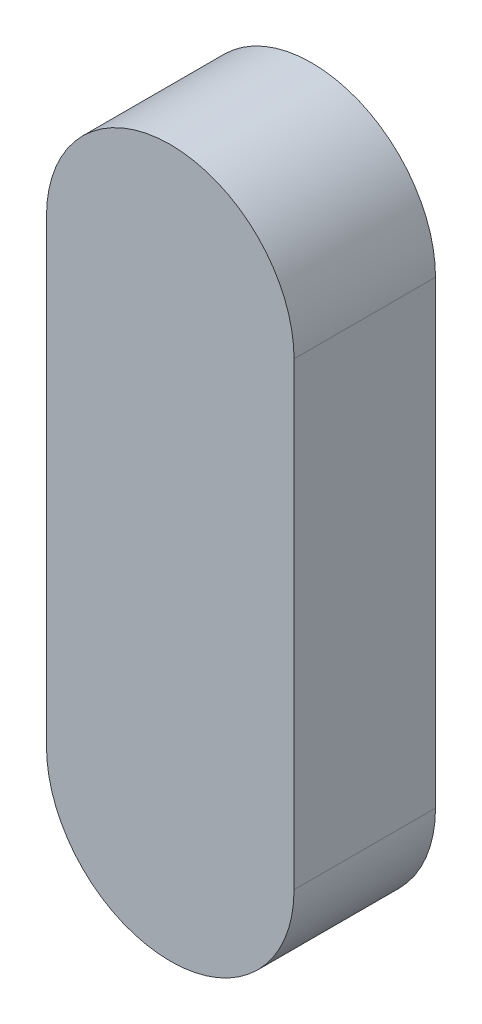
SolidWorks part; units mm, degrees
ref_plane "前视基准面" through (0, 0, 0) normal (0, 0, 1) x (1, 0, 0)
ref_plane "上视基准面" through (0, 0, 0) normal (0, 1, 0) x (1, 0, 0)
ref_plane "右视基准面" through (0, 0, 0) normal (1, 0, 0) x (0, 0, -1)
sketch "草图1" plane through (0, 0, 0) normal (0, 0, 1) x (1, 0, 0)
  line L0 (0, 0) -> (0, 104)
  line L1 (56, 104) -> (56, 0)
  arc A0 (0, 104) -> (56, 104) centre (28, 104) cw
  arc A1 (0, 0) -> (56, 0) centre (28, 0) ccw
extrude "凸台-拉伸1" add sketch "草图1" along normal blind 32 contours L0 A1 L1 A0
